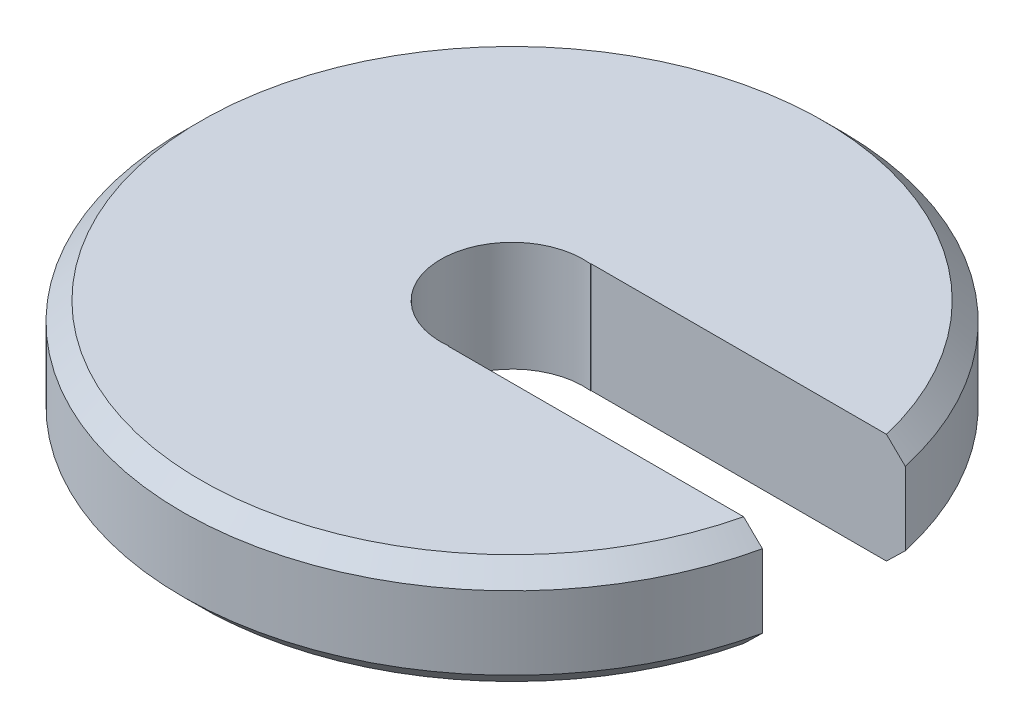
SolidWorks part; units mm, degrees
ref_plane "Front Plane" through (0, 0, 0) normal (0, 0, 1) x (1, 0, 0)
ref_plane "Top Plane" through (0, 0, 0) normal (0, 1, 0) x (1, 0, 0)
ref_plane "Right Plane" through (0, 0, 0) normal (1, 0, 0) x (0, 0, -1)
sketch "Sketch1" plane through (0, 0, 0) normal (0, 1, 0) x (1, 0, 0)
  circle A0 centre (0, 0) radius 30
  dimension "D1" = 60
extrude "Boss-Extrude1" add sketch "Sketch1" along normal blind 10
sketch "Sketch2" plane through (0, 10, 0) normal (0, 1, 0) x (1, 0, 0)
  line L0 (0, 0) -> (30, 0) construction
  line L1 (0.689, 6.5) -> (59.311, 6.5)
  line L2 (0.689, 6.5) -> (0.689, -6.5)
  line L3 (0.689, -6.5) -> (59.311, -6.5)
  line L4 (59.311, 6.5) -> (59.311, -6.5)
  line L5 (0.689, 6.5) -> (59.311, -6.5) construction
  line L6 (0.689, -6.5) -> (59.311, 6.5) construction
  circle A0 centre (0, 0) radius 30 construction
  point P0 (30, 0)
  dimension "D1" = 13
extrude "Cut-Extrude1" cut sketch "Sketch2" against normal blind 33
sketch "Sketch3" plane through (0, 10, 0) normal (0, 1, 0) x (1, 0, 0)
  circle A0 centre (0, 0) radius 6.5
  dimension "D1" = 13
extrude "Cut-Extrude2" cut sketch "Sketch3" against normal blind 33
chamfer "Chamfer1" distance 1.67 angle 45 2 edges at (-30, 0, 0) (-30, 10, 0)
